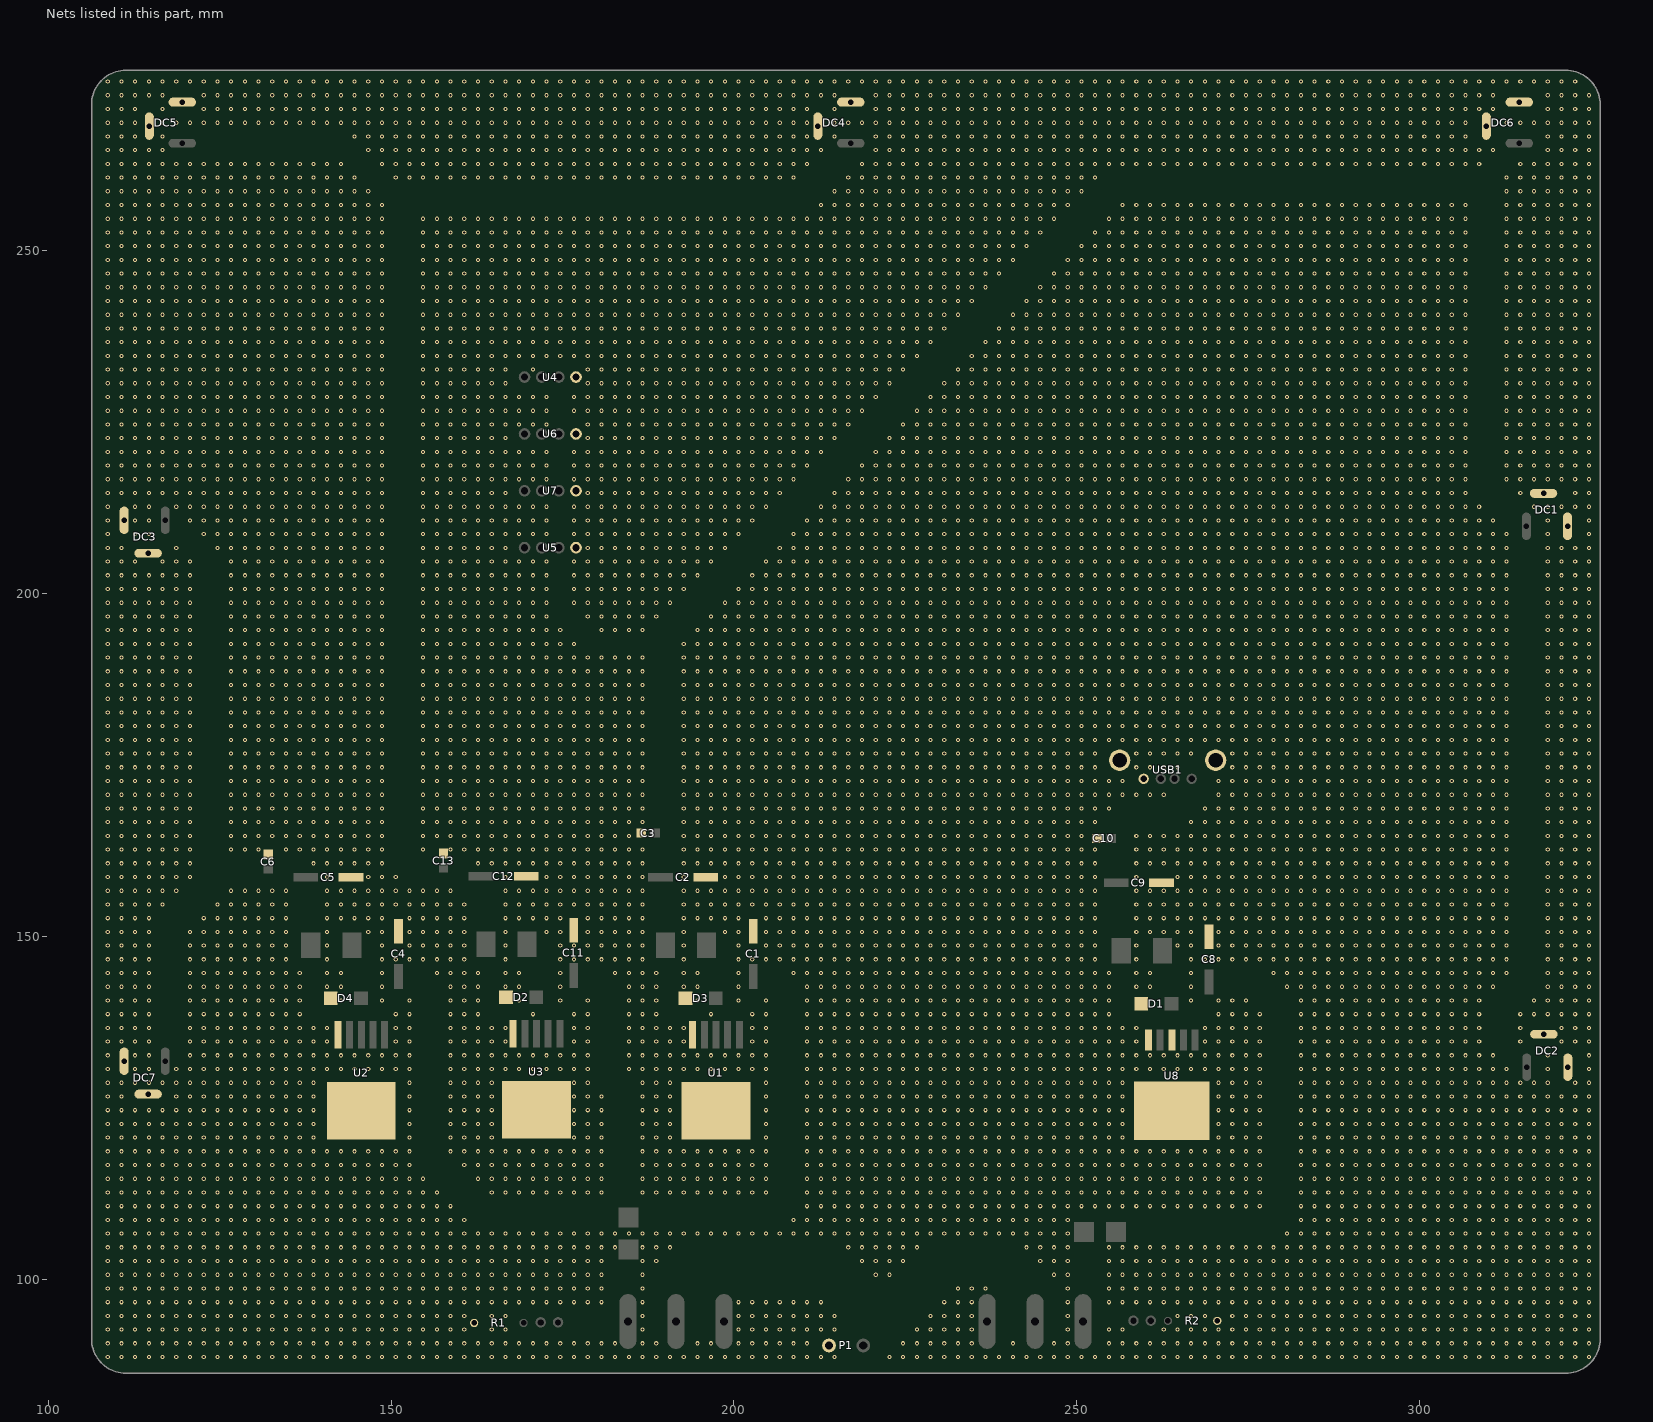
[diagram p0: the nets of this part, all layers, seen from the top]
# Altium PCB MISC49942.pcbdoc (part 4 of 4)
Units mm, origin at the board's own origin, x right, y up, seen from the top; angles counter-clockwise.
Board outline 220 x 190 mm, 2 copper layers (Top Layer, Bottom Layer), stack 1.58 mm thick; 45 components, 14 nets, 127 pads, 8689 vias.

## Via types
v1: diameter 0.61, hole 0.305, Top Layer to Bottom Layer, 8689 vias

## Nets (pads, with @x,y where several pads share a name; then routed paths per layer and width w, separated by ;. In a path a pad name is that pad's centre, name@x,y a point inside that pad or via, vN(x,y) a via of type N, cw(c..) or ccw(c..) an arc to the next point about the centre after c; other vN are vias at no path point) (continued)
GND: (continued)
  other v1: 204.684,220.669 206.684,220.669 208.684,220.669 210.684,220.669 212.684,220.669 220.684,220.669 222.684,220.669 224.684,220.669 226.684,220.669 228.684,220.669 230.684,220.669 232.684,220.669 234.684,220.669 236.684,220.669 238.684,220.669 240.684,220.669 242.684,220.669 244.684,220.669 246.684,220.669 248.684,220.669 250.684,220.669 252.684,220.669 254.684,220.669 256.684,220.669 258.684,220.669 260.684,220.669 262.684,220.669 264.684,220.669 266.684,220.669 268.684,220.669 270.684,220.669 272.684,220.669 274.684,220.669 276.684,220.669 278.684,220.669 280.684,220.669 282.684,220.669 284.684,220.669 286.684,220.669 288.684,220.669 290.684,220.669 292.684,220.669 294.684,220.669 296.684,220.669 298.684,220.669 300.684,220.669 302.684,220.669 304.684,220.669 306.684,220.669 312.684,220.669 314.684,220.669 316.684,220.669 318.684,220.669 320.684,220.669 322.684,220.669 324.684,220.669 108.684,222.669 110.684,222.669 112.684,222.669 114.684,222.669 116.684,222.669 118.684,222.669 120.684,222.669 122.684,222.669 124.684,222.669 126.684,222.669 128.684,222.669 130.684,222.669 132.684,222.669 134.684,222.669 136.684,222.669 138.684,222.669 140.684,222.669 142.684,222.669 144.684,222.669 146.684,222.669 148.684,222.669 154.684,222.669 156.684,222.669 158.684,222.669 160.684,222.669 162.684,222.669 164.684,222.669 166.684,222.669 178.684,222.669 180.684,222.669 182.684,222.669 184.684,222.669 186.684,222.669 188.684,222.669 190.684,222.669 192.684,222.669 194.684,222.669 196.684,222.669 198.684,222.669 200.684,222.669 202.684,222.669 204.684,222.669 206.684,222.669 208.684,222.669 210.684,222.669 212.684,222.669 214.684,222.669 222.684,222.669 224.684,222.669 226.684,222.669 228.684,222.669 230.684,222.669 232.684,222.669 234.684,222.669 236.684,222.669 238.684,222.669 240.684,222.669 242.684,222.669 244.684,222.669 246.684,222.669 248.684,222.669 250.684,222.669 252.684,222.669 254.684,222.669 256.684,222.669 258.684,222.669 260.684,222.669 262.684,222.669 264.684,222.669 266.684,222.669 268.684,222.669 270.684,222.669 272.684,222.669 274.684,222.669 276.684,222.669 278.684,222.669 280.684,222.669 282.684,222.669 284.684,222.669 286.684,222.669 288.684,222.669 290.684,222.669 292.684,222.669 294.684,222.669 296.684,222.669 298.684,222.669 300.684,222.669 302.684,222.669 304.684,222.669 306.684,222.669 312.684,222.669 314.684,222.669 316.684,222.669 318.684,222.669 320.684,222.669 322.684,222.669 324.684,222.669 108.684,224.669 110.684,224.669 112.684,224.669 114.684,224.669 116.684,224.669 118.684,224.669 120.684,224.669 122.684,224.669 124.684,224.669 126.684,224.669 128.684,224.669 130.684,224.669 132.684,224.669 134.684,224.669 136.684,224.669 138.684,224.669 140.684,224.669 142.684,224.669 144.684,224.669 146.684,224.669 148.684,224.669 154.684,224.669 156.684,224.669 158.684,224.669 160.684,224.669 162.684,224.669 164.684,224.669 166.684,224.669 168.684,224.669 170.684,224.669 172.684,224.669 178.684,224.669 180.684,224.669 182.684,224.669 184.684,224.669 186.684,224.669 188.684,224.669 190.684,224.669 192.684,224.669 194.684,224.669 196.684,224.669 198.684,224.669 200.684,224.669 202.684,224.669 204.684,224.669 206.684,224.669 208.684,224.669 210.684,224.669 212.684,224.669 214.684,224.669 216.684,224.669 224.684,224.669 226.684,224.669 228.684,224.669 230.684,224.669 232.684,224.669 234.684,224.669 236.684,224.669 238.684,224.669 240.684,224.669 242.684,224.669 244.684,224.669 246.684,224.669 248.684,224.669 250.684,224.669 252.684,224.669 254.684,224.669 256.684,224.669 258.684,224.669 260.684,224.669 262.684,224.669 264.684,224.669 266.684,224.669 268.684,224.669 270.684,224.669 272.684,224.669 274.684,224.669 276.684,224.669 278.684,224.669 280.684,224.669 282.684,224.669 284.684,224.669 286.684,224.669 288.684,224.669 290.684,224.669 292.684,224.669 294.684,224.669 296.684,224.669 298.684,224.669 300.684,224.669 302.684,224.669 304.684,224.669 306.684,224.669 312.684,224.669 314.684,224.669 316.684,224.669 318.684,224.669 320.684,224.669 322.684,224.669 324.684,224.669 108.684,226.669 110.684,226.669 112.684,226.669 114.684,226.669 116.684,226.669 118.684,226.669 120.684,226.669 122.684,226.669 124.684,226.669 126.684,226.669 128.684,226.669 130.684,226.669 132.684,226.669 134.684,226.669 136.684,226.669 138.684,226.669 140.684,226.669 142.684,226.669 144.684,226.669 146.684,226.669 148.684,226.669 154.684,226.669 156.684,226.669 158.684,226.669 160.684,226.669 162.684,226.669 164.684,226.669 166.684,226.669 168.684,226.669 170.684,226.669 172.684,226.669 176.684,226.669 178.684,226.669 180.684,226.669 182.684,226.669 184.684,226.669 186.684,226.669 188.684,226.669 190.684,226.669 192.684,226.669 194.684,226.669 196.684,226.669 198.684,226.669 200.684,226.669 202.684,226.669 204.684,226.669 206.684,226.669 208.684,226.669 210.684,226.669 212.684,226.669 214.684,226.669 216.684,226.669 218.684,226.669 226.684,226.669 228.684,226.669 230.684,226.669 232.684,226.669 234.684,226.669 236.684,226.669 238.684,226.669 240.684,226.669 242.684,226.669 244.684,226.669 246.684,226.669 248.684,226.669 250.684,226.669 252.684,226.669 254.684,226.669 256.684,226.669 258.684,226.669 260.684,226.669 262.684,226.669 264.684,226.669 266.684,226.669 268.684,226.669 270.684,226.669 272.684,226.669 274.684,226.669 276.684,226.669 278.684,226.669 280.684,226.669 282.684,226.669 284.684,226.669 286.684,226.669 288.684,226.669 290.684,226.669 292.684,226.669 294.684,226.669 296.684,226.669 298.684,226.669 300.684,226.669 302.684,226.669 304.684,226.669 306.684,226.669 312.684,226.669 314.684,226.669 316.684,226.669 318.684,226.669 320.684,226.669 322.684,226.669 324.684,226.669 108.684,228.669 110.684,228.669 112.684,228.669 114.684,228.669 116.684,228.669 118.684,228.669 120.684,228.669 122.684,228.669 124.684,228.669 126.684,228.669 128.684,228.669 130.684,228.669 132.684,228.669 134.684,228.669 136.684,228.669 138.684,228.669 140.684,228.669 142.684,228.669 144.684,228.669 146.684,228.669 148.684,228.669 154.684,228.669 156.684,228.669 158.684,228.669 160.684,228.669 162.684,228.669 164.684,228.669 166.684,228.669 168.684,228.669 170.684,228.669 172.684,228.669 176.684,228.669 178.684,228.669 180.684,228.669 182.684,228.669 184.684,228.669 186.684,228.669 188.684,228.669 190.684,228.669 192.684,228.669 194.684,228.669 196.684,228.669 198.684,228.669 200.684,228.669 202.684,228.669 204.684,228.669 206.684,228.669 208.684,228.669 210.684,228.669 212.684,228.669 214.684,228.669 216.684,228.669 218.684,228.669 220.684,228.669 228.684,228.669 230.684,228.669 232.684,228.669 234.684,228.669 236.684,228.669 238.684,228.669 240.684,228.669 242.684,228.669 244.684,228.669 246.684,228.669 248.684,228.669 250.684,228.669 252.684,228.669 254.684,228.669 256.684,228.669 258.684,228.669 260.684,228.669 262.684,228.669 264.684,228.669 266.684,228.669 268.684,228.669 270.684,228.669 272.684,228.669 274.684,228.669 276.684,228.669 278.684,228.669 280.684,228.669 282.684,228.669 284.684,228.669 286.684,228.669 288.684,228.669 290.684,228.669 292.684,228.669 294.684,228.669 296.684,228.669 298.684,228.669 300.684,228.669 302.684,228.669 304.684,228.669 306.684,228.669 312.684,228.669 314.684,228.669 316.684,228.669 318.684,228.669 320.684,228.669 322.684,228.669 324.684,228.669 108.684,230.669 110.684,230.669 112.684,230.669 114.684,230.669 116.684,230.669 118.684,230.669 120.684,230.669 122.684,230.669 124.684,230.669 126.684,230.669 128.684,230.669 130.684,230.669 132.684,230.669 134.684,230.669 136.684,230.669 138.684,230.669 140.684,230.669 142.684,230.669 144.684,230.669 146.684,230.669 148.684,230.669 154.684,230.669 156.684,230.669 158.684,230.669 160.684,230.669 162.684,230.669 164.684,230.669 166.684,230.669 178.684,230.669 180.684,230.669 182.684,230.669 184.684,230.669 186.684,230.669 188.684,230.669 190.684,230.669 192.684,230.669 194.684,230.669 196.684,230.669 198.684,230.669 200.684,230.669 202.684,230.669 204.684,230.669 206.684,230.669 208.684,230.669 210.684,230.669 212.684,230.669 214.684,230.669 216.684,230.669 218.684,230.669 220.684,230.669 222.684,230.669 230.684,230.669 232.684,230.669 234.684,230.669 236.684,230.669 238.684,230.669 240.684,230.669 242.684,230.669 244.684,230.669 246.684,230.669 248.684,230.669 250.684,230.669 252.684,230.669 254.684,230.669 256.684,230.669 258.684,230.669 260.684,230.669 262.684,230.669 264.684,230.669 266.684,230.669 268.684,230.669 270.684,230.669 272.684,230.669 274.684,230.669 276.684,230.669 278.684,230.669 280.684,230.669 282.684,230.669 284.684,230.669 286.684,230.669 288.684,230.669 290.684,230.669 292.684,230.669 294.684,230.669 296.684,230.669 298.684,230.669 300.684,230.669 302.684,230.669 304.684,230.669 306.684,230.669 312.684,230.669 314.684,230.669 316.684,230.669 318.684,230.669 320.684,230.669 322.684,230.669 324.684,230.669 108.684,232.669 110.684,232.669 112.684,232.669 114.684,232.669 116.684,232.669 118.684,232.669 120.684,232.669 122.684,232.669 124.684,232.669 126.684,232.669 128.684,232.669 130.684,232.669 132.684,232.669 134.684,232.669 136.684,232.669 138.684,232.669 140.684,232.669 142.684,232.669 144.684,232.669 146.684,232.669 148.684,232.669 154.684,232.669 156.684,232.669 158.684,232.669 160.684,232.669 162.684,232.669 164.684,232.669 166.684,232.669 170.684,232.669 178.684,232.669 180.684,232.669 182.684,232.669 184.684,232.669 186.684,232.669 188.684,232.669 190.684,232.669 192.684,232.669 194.684,232.669 196.684,232.669 198.684,232.669 200.684,232.669 202.684,232.669 204.684,232.669 206.684,232.669 208.684,232.669 210.684,232.669 212.684,232.669 214.684,232.669 216.684,232.669 218.684,232.669 220.684,232.669 222.684,232.669 224.684,232.669 232.684,232.669 234.684,232.669 236.684,232.669 238.684,232.669 240.684,232.669 242.684,232.669 244.684,232.669 246.684,232.669 248.684,232.669 250.684,232.669 252.684,232.669 254.684,232.669 256.684,232.669 258.684,232.669 260.684,232.669 262.684,232.669 264.684,232.669 266.684,232.669 268.684,232.669 270.684,232.669 272.684,232.669 274.684,232.669 276.684,232.669 278.684,232.669 280.684,232.669 282.684,232.669 284.684,232.669 286.684,232.669 288.684,232.669 290.684,232.669 292.684,232.669 294.684,232.669 296.684,232.669 298.684,232.669 300.684,232.669 302.684,232.669 304.684,232.669 306.684,232.669 312.684,232.669 314.684,232.669 316.684,232.669 318.684,232.669 320.684,232.669 322.684,232.669 324.684,232.669 108.684,234.669 110.684,234.669 112.684,234.669 114.684,234.669 116.684,234.669 118.684,234.669 120.684,234.669 122.684,234.669 124.684,234.669 126.684,234.669 128.684,234.669 130.684,234.669 132.684,234.669 134.684,234.669 136.684,234.669 138.684,234.669 140.684,234.669 142.684,234.669 144.684,234.669 146.684,234.669 148.684,234.669 154.684,234.669 156.684,234.669 158.684,234.669 160.684,234.669 162.684,234.669 164.684,234.669 166.684,234.669 168.684,234.669 170.684,234.669 172.684,234.669 174.684,234.669 176.684,234.669 178.684,234.669 180.684,234.669 182.684,234.669 184.684,234.669 186.684,234.669 188.684,234.669 190.684,234.669 192.684,234.669 194.684,234.669 196.684,234.669 198.684,234.669 200.684,234.669 202.684,234.669 204.684,234.669 206.684,234.669 208.684,234.669 210.684,234.669 212.684,234.669 214.684,234.669 216.684,234.669 218.684,234.669 220.684,234.669 222.684,234.669 224.684,234.669 226.684,234.669 234.684,234.669 236.684,234.669 238.684,234.669 240.684,234.669 242.684,234.669 244.684,234.669 246.684,234.669 248.684,234.669 250.684,234.669 252.684,234.669 254.684,234.669 256.684,234.669 258.684,234.669 260.684,234.669 262.684,234.669 264.684,234.669 266.684,234.669 268.684,234.669 270.684,234.669 272.684,234.669 274.684,234.669 276.684,234.669 278.684,234.669 280.684,234.669 282.684,234.669 284.684,234.669 286.684,234.669 288.684,234.669 290.684,234.669 292.684,234.669 294.684,234.669 296.684,234.669 298.684,234.669 300.684,234.669 302.684,234.669 304.684,234.669 306.684,234.669 312.684,234.669 314.684,234.669 316.684,234.669 318.684,234.669 320.684,234.669 322.684,234.669 324.684,234.669 108.684,236.669 110.684,236.669 112.684,236.669 114.684,236.669 116.684,236.669 118.684,236.669 120.684,236.669 122.684,236.669 124.684,236.669 126.684,236.669 128.684,236.669 130.684,236.669 132.684,236.669 134.684,236.669 136.684,236.669 138.684,236.669 140.684,236.669 142.684,236.669 144.684,236.669 146.684,236.669 148.684,236.669 154.684,236.669 156.684,236.669 158.684,236.669 160.684,236.669 162.684,236.669 164.684,236.669 166.684,236.669 168.684,236.669 170.684,236.669 172.684,236.669 174.684,236.669 176.684,236.669 178.684,236.669 180.684,236.669 182.684,236.669 184.684,236.669 186.684,236.669 188.684,236.669 190.684,236.669 192.684,236.669 194.684,236.669 196.684,236.669 198.684,236.669 200.684,236.669 202.684,236.669 204.684,236.669 206.684,236.669 208.684,236.669 210.684,236.669 212.684,236.669 214.684,236.669 216.684,236.669 218.684,236.669 220.684,236.669 222.684,236.669 224.684,236.669 226.684,236.669 228.684,236.669 236.684,236.669 238.684,236.669 240.684,236.669 242.684,236.669 244.684,236.669 246.684,236.669 248.684,236.669 250.684,236.669 252.684,236.669 254.684,236.669 256.684,236.669 258.684,236.669 260.684,236.669 262.684,236.669 264.684,236.669 266.684,236.669 268.684,236.669 270.684,236.669 272.684,236.669 274.684,236.669 276.684,236.669 278.684,236.669 280.684,236.669 282.684,236.669 284.684,236.669 286.684,236.669 288.684,236.669 290.684,236.669 292.684,236.669 294.684,236.669 296.684,236.669 298.684,236.669 300.684,236.669 302.684,236.669 304.684,236.669 306.684,236.669 312.684,236.669 314.684,236.669 316.684,236.669 318.684,236.669 320.684,236.669 322.684,236.669 324.684,236.669 108.684,238.669 110.684,238.669 112.684,238.669 114.684,238.669 116.684,238.669 118.684,238.669 120.684,238.669 122.684,238.669 124.684,238.669 126.684,238.669 128.684,238.669 130.684,238.669 132.684,238.669 134.684,238.669 136.684,238.669 138.684,238.669 140.684,238.669 142.684,238.669 144.684,238.669 146.684,238.669 148.684,238.669 154.684,238.669 156.684,238.669 158.684,238.669 160.684,238.669 162.684,238.669 164.684,238.669 166.684,238.669 168.684,238.669 170.684,238.669 172.684,238.669 174.684,238.669 176.684,238.669 178.684,238.669 180.684,238.669 182.684,238.669 184.684,238.669 186.684,238.669 188.684,238.669 190.684,238.669 192.684,238.669 194.684,238.669 196.684,238.669 198.684,238.669 200.684,238.669 202.684,238.669 204.684,238.669 206.684,238.669 208.684,238.669 210.684,238.669 212.684,238.669 214.684,238.669 216.684,238.669 218.684,238.669 220.684,238.669 222.684,238.669 224.684,238.669 226.684,238.669 228.684,238.669 230.684,238.669 238.684,238.669 240.684,238.669 242.684,238.669 244.684,238.669 246.684,238.669 248.684,238.669 250.684,238.669 252.684,238.669 254.684,238.669 256.684,238.669 258.684,238.669 260.684,238.669 262.684,238.669 264.684,238.669 266.684,238.669 268.684,238.669 270.684,238.669 272.684,238.669 274.684,238.669 276.684,238.669 278.684,238.669 280.684,238.669 282.684,238.669 284.684,238.669 286.684,238.669 288.684,238.669 290.684,238.669 292.684,238.669 294.684,238.669 296.684,238.669 298.684,238.669 300.684,238.669 302.684,238.669 304.684,238.669 306.684,238.669 312.684,238.669 314.684,238.669 316.684,238.669 318.684,238.669 320.684,238.669 322.684,238.669 324.684,238.669 108.684,240.669 110.684,240.669 112.684,240.669 114.684,240.669 116.684,240.669 118.684,240.669 120.684,240.669 122.684,240.669 124.684,240.669 126.684,240.669 128.684,240.669 130.684,240.669 132.684,240.669 134.684,240.669 136.684,240.669 138.684,240.669 140.684,240.669 142.684,240.669 144.684,240.669 146.684,240.669 148.684,240.669 154.684,240.669 156.684,240.669 158.684,240.669 160.684,240.669 162.684,240.669 164.684,240.669 166.684,240.669 168.684,240.669 170.684,240.669 172.684,240.669 174.684,240.669 176.684,240.669 178.684,240.669 180.684,240.669 182.684,240.669 184.684,240.669 186.684,240.669 188.684,240.669 190.684,240.669 192.684,240.669 194.684,240.669 196.684,240.669 198.684,240.669 200.684,240.669 202.684,240.669 204.684,240.669 206.684,240.669 208.684,240.669 210.684,240.669 212.684,240.669 214.684,240.669 216.684,240.669 218.684,240.669 220.684,240.669 222.684,240.669 224.684,240.669 226.684,240.669 228.684,240.669 230.684,240.669 232.684,240.669 240.684,240.669 242.684,240.669 244.684,240.669 246.684,240.669 248.684,240.669 250.684,240.669 252.684,240.669 254.684,240.669 256.684,240.669 258.684,240.669 260.684,240.669 262.684,240.669 264.684,240.669 266.684,240.669 268.684,240.669 270.684,240.669 272.684,240.669 274.684,240.669 276.684,240.669 278.684,240.669 280.684,240.669 282.684,240.669 284.684,240.669 286.684,240.669 288.684,240.669 290.684,240.669 292.684,240.669 294.684,240.669 296.684,240.669 298.684,240.669 300.684,240.669 302.684,240.669 304.684,240.669 306.684,240.669 312.684,240.669 314.684,240.669 316.684,240.669 318.684,240.669 320.684,240.669 322.684,240.669 324.684,240.669 108.684,242.669 110.684,242.669 112.684,242.669 114.684,242.669 116.684,242.669 118.684,242.669 120.684,242.669 122.684,242.669 124.684,242.669 126.684,242.669 128.684,242.669 130.684,242.669 132.684,242.669 134.684,242.669 136.684,242.669 138.684,242.669 140.684,242.669 142.684,242.669 144.684,242.669 146.684,242.669 148.684,242.669 154.684,242.669 156.684,242.669 158.684,242.669 160.684,242.669 162.684,242.669 164.684,242.669 166.684,242.669 168.684,242.669 170.684,242.669 172.684,242.669 174.684,242.669 176.684,242.669 178.684,242.669 180.684,242.669 182.684,242.669 184.684,242.669 186.684,242.669 188.684,242.669 190.684,242.669 192.684,242.669 194.684,242.669 196.684,242.669 198.684,242.669 200.684,242.669 202.684,242.669 204.684,242.669 206.684,242.669 208.684,242.669 210.684,242.669 212.684,242.669 214.684,242.669 216.684,242.669 218.684,242.669 220.684,242.669 222.684,242.669 224.684,242.669 226.684,242.669 228.684,242.669 230.684,242.669 232.684,242.669 234.684,242.669 242.684,242.669 244.684,242.669 246.684,242.669 248.684,242.669 250.684,242.669 252.684,242.669 254.684,242.669 256.684,242.669 258.684,242.669 260.684,242.669 262.684,242.669 264.684,242.669 266.684,242.669 268.684,242.669 270.684,242.669 272.684,242.669 274.684,242.669 276.684,242.669 278.684,242.669 280.684,242.669 282.684,242.669 284.684,242.669 286.684,242.669 288.684,242.669 290.684,242.669 292.684,242.669 294.684,242.669 296.684,242.669 298.684,242.669 300.684,242.669 302.684,242.669 304.684,242.669 306.684,242.669 312.684,242.669 314.684,242.669 316.684,242.669 318.684,242.669 320.684,242.669 322.684,242.669 324.684,242.669 108.684,244.669 110.684,244.669 112.684,244.669 114.684,244.669 116.684,244.669 118.684,244.669 120.684,244.669 122.684,244.669 124.684,244.669 126.684,244.669 128.684,244.669 130.684,244.669 132.684,244.669 134.684,244.669 136.684,244.669 138.684,244.669 140.684,244.669 142.684,244.669 144.684,244.669 146.684,244.669 148.684,244.669 154.684,244.669 156.684,244.669 158.684,244.669 160.684,244.669 162.684,244.669 164.684,244.669 166.684,244.669 168.684,244.669 170.684,244.669 172.684,244.669 174.684,244.669 176.684,244.669 178.684,244.669 180.684,244.669 182.684,244.669 184.684,244.669 186.684,244.669 188.684,244.669 190.684,244.669 192.684,244.669 194.684,244.669 196.684,244.669 198.684,244.669 200.684,244.669 202.684,244.669 204.684,244.669 206.684,244.669 208.684,244.669 210.684,244.669 212.684,244.669 214.684,244.669 216.684,244.669 218.684,244.669 220.684,244.669 222.684,244.669 224.684,244.669 226.684,244.669 228.684,244.669 230.684,244.669 232.684,244.669 234.684,244.669 236.684,244.669 244.684,244.669 246.684,244.669 248.684,244.669 250.684,244.669 252.684,244.669 254.684,244.669 256.684,244.669 258.684,244.669 260.684,244.669 262.684,244.669 264.684,244.669 266.684,244.669 268.684,244.669 270.684,244.669 272.684,244.669 274.684,244.669 276.684,244.669 278.684,244.669 280.684,244.669 282.684,244.669 284.684,244.669 286.684,244.669 288.684,244.669 290.684,244.669 292.684,244.669 294.684,244.669 296.684,244.669 298.684,244.669 300.684,244.669 302.684,244.669 304.684,244.669 306.684,244.669 312.684,244.669 314.684,244.669 316.684,244.669 318.684,244.669 320.684,244.669 322.684,244.669 324.684,244.669 108.684,246.669 110.684,246.669 112.684,246.669 114.684,246.669 116.684,246.669 118.684,246.669 120.684,246.669 122.684,246.669 124.684,246.669 126.684,246.669 128.684,246.669 130.684,246.669 132.684,246.669 134.684,246.669 136.684,246.669 138.684,246.669 140.684,246.669 142.684,246.669 144.684,246.669 146.684,246.669 148.684,246.669 154.684,246.669 156.684,246.669 158.684,246.669 160.684,246.669 162.684,246.669 164.684,246.669 166.684,246.669 168.684,246.669 170.684,246.669 172.684,246.669 174.684,246.669 176.684,246.669 178.684,246.669 180.684,246.669 182.684,246.669 184.684,246.669 186.684,246.669 188.684,246.669 190.684,246.669 192.684,246.669 194.684,246.669 196.684,246.669 198.684,246.669 200.684,246.669 202.684,246.669 204.684,246.669 206.684,246.669 208.684,246.669 210.684,246.669 212.684,246.669 214.684,246.669 216.684,246.669 218.684,246.669 220.684,246.669 222.684,246.669 224.684,246.669 226.684,246.669 228.684,246.669 230.684,246.669 232.684,246.669 234.684,246.669 236.684,246.669 238.684,246.669 246.684,246.669 248.684,246.669 250.684,246.669 252.684,246.669 254.684,246.669 256.684,246.669 258.684,246.669 260.684,246.669 262.684,246.669 264.684,246.669 266.684,246.669 268.684,246.669 270.684,246.669 272.684,246.669 274.684,246.669 276.684,246.669 278.684,246.669 280.684,246.669 282.684,246.669 284.684,246.669 286.684,246.669 288.684,246.669 290.684,246.669 292.684,246.669 294.684,246.669 296.684,246.669 298.684,246.669 300.684,246.669 302.684,246.669 304.684,246.669 306.684,246.669 312.684,246.669 314.684,246.669 316.684,246.669 318.684,246.669 320.684,246.669 322.684,246.669 324.684,246.669 108.684,248.669 110.684,248.669 112.684,248.669 114.684,248.669 116.684,248.669 118.684,248.669 120.684,248.669 122.684,248.669 124.684,248.669 126.684,248.669 128.684,248.669 130.684,248.669 132.684,248.669 134.684,248.669 136.684,248.669 138.684,248.669 140.684,248.669 142.684,248.669 144.684,248.669 146.684,248.669 148.684,248.669 154.684,248.669 156.684,248.669 158.684,248.669 160.684,248.669 162.684,248.669 164.684,248.669 166.684,248.669 168.684,248.669 170.684,248.669 172.684,248.669 174.684,248.669 176.684,248.669 178.684,248.669 180.684,248.669 182.684,248.669 184.684,248.669 186.684,248.669 188.684,248.669 190.684,248.669 192.684,248.669 194.684,248.669 196.684,248.669 198.684,248.669 200.684,248.669 202.684,248.669 204.684,248.669 206.684,248.669 208.684,248.669 210.684,248.669 212.684,248.669 214.684,248.669 216.684,248.669 218.684,248.669 220.684,248.669 222.684,248.669 224.684,248.669 226.684,248.669 228.684,248.669 230.684,248.669 232.684,248.669 234.684,248.669 236.684,248.669 238.684,248.669 240.684,248.669 248.684,248.669 250.684,248.669 252.684,248.669 254.684,248.669 256.684,248.669 258.684,248.669 260.684,248.669 262.684,248.669 264.684,248.669 266.684,248.669 268.684,248.669 270.684,248.669 272.684,248.669 274.684,248.669 276.684,248.669 278.684,248.669 280.684,248.669 282.684,248.669 284.684,248.669 286.684,248.669 288.684,248.669 290.684,248.669 292.684,248.669 294.684,248.669 296.684,248.669 298.684,248.669 300.684,248.669 302.684,248.669 304.684,248.669 306.684,248.669 312.684,248.669 314.684,248.669 316.684,248.669 318.684,248.669 320.684,248.669 322.684,248.669 324.684,248.669 108.684,250.669 110.684,250.669 112.684,250.669 114.684,250.669 116.684,250.669 118.684,250.669 120.684,250.669 122.684,250.669 124.684,250.669 126.684,250.669 128.684,250.669 130.684,250.669 132.684,250.669 134.684,250.669 136.684,250.669 138.684,250.669 140.684,250.669 142.684,250.669 144.684,250.669 146.684,250.669 148.684,250.669 154.684,250.669 156.684,250.669 158.684,250.669 160.684,250.669 162.684,250.669 164.684,250.669 166.684,250.669 168.684,250.669 170.684,250.669 172.684,250.669 174.684,250.669 176.684,250.669 178.684,250.669 180.684,250.669 182.684,250.669 184.684,250.669 186.684,250.669 188.684,250.669 190.684,250.669 192.684,250.669 194.684,250.669 196.684,250.669 198.684,250.669 200.684,250.669 202.684,250.669 204.684,250.669 206.684,250.669 208.684,250.669 210.684,250.669 212.684,250.669 214.684,250.669 216.684,250.669 218.684,250.669 220.684,250.669 222.684,250.669 224.684,250.669 226.684,250.669 228.684,250.669 230.684,250.669 232.684,250.669 234.684,250.669 236.684,250.669 238.684,250.669 240.684,250.669 242.684,250.669 250.684,250.669 252.684,250.669 254.684,250.669 256.684,250.669 258.684,250.669 260.684,250.669 262.684,250.669 264.684,250.669 266.684,250.669 268.684,250.669 270.684,250.669 272.684,250.669 274.684,250.669 276.684,250.669 278.684,250.669 280.684,250.669 282.684,250.669 284.684,250.669 286.684,250.669 288.684,250.669 290.684,250.669 292.684,250.669 294.684,250.669 296.684,250.669 298.684,250.669 300.684,250.669 302.684,250.669 304.684,250.669 306.684,250.669 312.684,250.669 314.684,250.669 316.684,250.669 318.684,250.669 320.684,250.669 322.684,250.669 324.684,250.669 108.684,252.669 110.684,252.669 112.684,252.669 114.684,252.669 116.684,252.669 118.684,252.669 120.684,252.669 122.684,252.669 124.684,252.669 126.684,252.669 128.684,252.669 130.684,252.669 132.684,252.669 134.684,252.669 136.684,252.669 138.684,252.669 140.684,252.669 142.684,252.669 144.684,252.669 146.684,252.669 148.684,252.669 154.684,252.669 156.684,252.669 158.684,252.669 160.684,252.669 162.684,252.669 164.684,252.669 166.684,252.669 168.684,252.669 170.684,252.669 172.684,252.669 174.684,252.669 176.684,252.669 178.684,252.669 180.684,252.669 182.684,252.669 184.684,252.669 186.684,252.669 188.684,252.669 190.684,252.669 192.684,252.669 194.684,252.669 196.684,252.669 198.684,252.669 200.684,252.669 202.684,252.669 204.684,252.669 206.684,252.669 208.684,252.669 210.684,252.669 212.684,252.669 214.684,252.669 216.684,252.669 218.684,252.669 220.684,252.669 222.684,252.669 224.684,252.669 226.684,252.669 228.684,252.669 230.684,252.669 232.684,252.669 234.684,252.669 236.684,252.669 238.684,252.669 240.684,252.669 242.684,252.669 244.684,252.669 252.684,252.669 254.684,252.669 256.684,252.669 258.684,252.669 260.684,252.669 262.684,252.669 264.684,252.669 266.684,252.669 268.684,252.669 270.684,252.669 272.684,252.669 274.684,252.669 276.684,252.669 278.684,252.669 280.684,252.669 282.684,252.669 284.684,252.669 286.684,252.669 288.684,252.669 290.684,252.669 292.684,252.669 294.684,252.669 296.684,252.669 298.684,252.669 300.684,252.669 302.684,252.669 304.684,252.669 306.684,252.669 312.684,252.669 314.684,252.669 316.684,252.669 318.684,252.669 320.684,252.669 322.684,252.669 324.684,252.669 108.684,254.669 110.684,254.669 112.684,254.669 114.684,254.669 116.684,254.669 118.684,254.669 120.684,254.669 122.684,254.669 124.684,254.669 126.684,254.669 128.684,254.669 130.684,254.669 132.684,254.669 134.684,254.669 136.684,254.669 138.684,254.669 140.684,254.669 142.684,254.669 144.684,254.669 146.684,254.669 148.684,254.669 154.684,254.669 156.684,254.669 158.684,254.669 160.684,254.669 162.684,254.669 164.684,254.669 166.684,254.669 168.684,254.669 170.684,254.669 172.684,254.669 174.684,254.669 176.684,254.669 178.684,254.669 180.684,254.669 182.684,254.669 184.684,254.669 186.684,254.669 188.684,254.669 190.684,254.669 192.684,254.669 194.684,254.669 196.684,254.669 198.684,254.669 200.684,254.669 202.684,254.669 204.684,254.669 206.684,254.669 208.684,254.669 210.684,254.669 212.684,254.669 214.684,254.669 216.684,254.669 218.684,254.669 220.684,254.669 222.684,254.669 224.684,254.669 226.684,254.669 228.684,254.669 230.684,254.669 232.684,254.669 234.684,254.669 236.684,254.669 238.684,254.669 240.684,254.669 242.684,254.669 244.684,254.669 246.684,254.669 254.684,254.669 256.684,254.669 258.684,254.669 260.684,254.669 262.684,254.669 264.684,254.669 266.684,254.669 268.684,254.669 270.684,254.669 272.684,254.669 274.684,254.669 276.684,254.669 278.684,254.669 280.684,254.669 282.684,254.669 284.684,254.669 286.684,254.669 288.684,254.669 290.684,254.669 292.684,254.669 294.684,254.669 296.684,254.669 298.684,254.669 300.684,254.669 302.684,254.669 304.684,254.669 306.684,254.669 312.684,254.669 314.684,254.669 316.684,254.669 318.684,254.669 320.684,254.669 322.684,254.669 324.684,254.669 108.684,256.669 110.684,256.669 112.684,256.669 114.684,256.669 116.684,256.669 118.684,256.669 120.684,256.669 122.684,256.669 124.684,256.669 126.684,256.669 128.684,256.669 130.684,256.669 132.684,256.669 134.684,256.669 136.684,256.669 138.684,256.669 140.684,256.669 142.684,256.669 144.684,256.669 146.684,256.669 148.684,256.669 212.684,256.669 214.684,256.669 216.684,256.669 218.684,256.669 220.684,256.669 222.684,256.669 224.684,256.669 226.684,256.669 228.684,256.669 230.684,256.669 232.684,256.669 234.684,256.669 236.684,256.669 238.684,256.669 240.684,256.669 242.684,256.669 244.684,256.669 246.684,256.669 248.684,256.669 256.684,256.669 258.684,256.669 260.684,256.669 262.684,256.669 264.684,256.669 266.684,256.669 268.684,256.669 270.684,256.669 272.684,256.669 274.684,256.669 276.684,256.669 278.684,256.669 280.684,256.669 282.684,256.669 284.684,256.669 286.684,256.669 288.684,256.669 290.684,256.669 292.684,256.669 294.684,256.669 296.684,256.669 298.684,256.669 300.684,256.669 302.684,256.669 304.684,256.669 306.684,256.669 312.684,256.669 314.684,256.669 316.684,256.669 318.684,256.669 320.684,256.669 322.684,256.669 324.684,256.669 108.684,258.669 110.684,258.669 112.684,258.669 114.684,258.669 116.684,258.669 118.684,258.669 120.684,258.669 122.684,258.669 124.684,258.669 126.684,258.669 128.684,258.669 130.684,258.669 132.684,258.669 134.684,258.669 136.684,258.669 138.684,258.669 140.684,258.669 142.684,258.669 144.684,258.669 146.684,258.669 214.684,258.669 216.684,258.669 218.684,258.669 220.684,258.669 222.684,258.669 224.684,258.669 226.684,258.669 228.684,258.669 230.684,258.669 232.684,258.669 234.684,258.669 236.684,258.669 238.684,258.669 240.684,258.669 242.684,258.669 244.684,258.669 246.684,258.669 248.684,258.669 250.684,258.669 312.684,258.669 314.684,258.669 316.684,258.669 318.684,258.669 320.684,258.669 322.684,258.669 324.684,258.669 108.684,260.669 110.684,260.669 112.684,260.669 114.684,260.669 116.684,260.669 118.684,260.669 120.684,260.669 122.684,260.669 124.684,260.669 126.684,260.669 128.684,260.669 130.684,260.669 132.684,260.669 134.684,260.669 136.684,260.669 138.684,260.669 140.684,260.669 142.684,260.669 144.684,260.669 150.684,260.669 152.684,260.669 154.684,260.669 156.684,260.669 158.684,260.669 160.684,260.669 162.684,260.669 164.684,260.669 166.684,260.669 168.684,260.669 170.684,260.669 172.684,260.669 174.684,260.669 176.684,260.669 178.684,260.669 180.684,260.669 182.684,260.669 184.684,260.669 186.684,260.669 188.684,260.669 190.684,260.669 192.684,260.669 194.684,260.669 196.684,260.669 198.684,260.669 200.684,260.669 202.684,260.669 204.684,260.669 206.684,260.669 208.684,260.669 216.684,260.669 218.684,260.669 220.684,260.669 222.684,260.669 224.684,260.669 226.684,260.669 228.684,260.669 230.684,260.669 232.684,260.669 234.684,260.669 236.684,260.669 238.684,260.669 240.684,260.669 242.684,260.669 244.684,260.669 246.684,260.669 248.684,260.669 250.684,260.669 252.684,260.669 312.684,260.669 314.684,260.669 316.684,260.669 318.684,260.669 320.684,260.669 322.684,260.669 324.684,260.669 108.684,262.669 110.684,262.669 112.684,262.669 114.684,262.669 116.684,262.669 118.684,262.669 120.684,262.669 122.684,262.669 124.684,262.669 126.684,262.669 128.684,262.669 130.684,262.669 132.684,262.669 134.684,262.669 136.684,262.669 138.684,262.669 140.684,262.669 142.684,262.669 148.684,262.669 150.684,262.669 152.684,262.669 154.684,262.669 156.684,262.669 158.684,262.669 160.684,262.669 162.684,262.669 164.684,262.669 166.684,262.669 168.684,262.669 170.684,262.669 172.684,262.669 174.684,262.669 176.684,262.669 178.684,262.669 180.684,262.669 182.684,262.669 184.684,262.669 186.684,262.669 188.684,262.669 190.684,262.669 192.684,262.669 194.684,262.669 196.684,262.669 198.684,262.669 200.684,262.669 202.684,262.669 204.684,262.669 206.684,262.669 208.684,262.669 210.684,262.669 218.684,262.669 220.684,262.669 222.684,262.669 224.684,262.669 226.684,262.669 228.684,262.669 230.684,262.669 232.684,262.669 234.684,262.669 236.684,262.669 238.684,262.669 240.684,262.669 242.684,262.669 244.684,262.669 246.684,262.669 248.684,262.669 250.684,262.669 252.684,262.669 254.684,262.669 256.684,262.669 258.684,262.669 260.684,262.669 262.684,262.669 264.684,262.669 266.684,262.669 268.684,262.669 270.684,262.669 272.684,262.669 274.684,262.669 276.684,262.669 278.684,262.669 280.684,262.669 282.684,262.669 284.684,262.669 286.684,262.669 288.684,262.669 290.684,262.669 292.684,262.669 294.684,262.669 296.684,262.669 298.684,262.669 300.684,262.669 302.684,262.669 304.684,262.669 306.684,262.669 308.684,262.669 314.684,262.669 316.684,262.669 318.684,262.669 320.684,262.669 322.684,262.669 324.684,262.669 108.684,264.669 110.684,264.669 112.684,264.669 114.684,264.669 116.684,264.669 146.684,264.669 148.684,264.669 150.684,264.669 152.684,264.669 154.684,264.669 156.684,264.669 158.684,264.669 160.684,264.669 162.684,264.669 164.684,264.669 166.684,264.669 168.684,264.669 170.684,264.669 172.684,264.669 174.684,264.669 176.684,264.669 178.684,264.669 180.684,264.669 182.684,264.669 184.684,264.669 186.684,264.669 188.684,264.669 190.684,264.669 192.684,264.669 194.684,264.669 196.684,264.669 198.684,264.669 200.684,264.669 202.684,264.669 204.684,264.669 206.684,264.669 208.684,264.669 210.684,264.669 212.684,264.669 220.684,264.669 222.684,264.669 224.684,264.669 226.684,264.669 228.684,264.669 230.684,264.669 232.684,264.669 234.684,264.669 236.684,264.669 238.684,264.669 240.684,264.669 242.684,264.669 244.684,264.669 246.684,264.669 248.684,264.669 250.684,264.669 252.684,264.669 254.684,264.669 256.684,264.669 258.684,264.669 260.684,264.669 262.684,264.669 264.684,264.669 266.684,264.669 268.684,264.669 270.684,264.669 272.684,264.669 274.684,264.669 276.684,264.669 278.684,264.669 280.684,264.669 282.684,264.669 284.684,264.669 286.684,264.669 288.684,264.669 290.684,264.669 292.684,264.669 294.684,264.669 296.684,264.669 298.684,264.669 300.684,264.669 302.684,264.669 304.684,264.669 306.684,264.669 308.684,264.669 310.684,264.669 318.684,264.669 320.684,264.669 322.684,264.669 324.684,264.669 108.684,266.669 110.684,266.669 112.684,266.669 116.684,266.669 144.684,266.669 146.684,266.669 148.684,266.669 150.684,266.669 152.684,266.669 154.684,266.669 156.684,266.669 158.684,266.669 160.684,266.669 162.684,266.669 164.684,266.669 166.684,266.669 168.684,266.669 170.684,266.669 172.684,266.669 174.684,266.669 176.684,266.669 178.684,266.669 180.684,266.669 182.684,266.669 184.684,266.669 186.684,266.669 188.684,266.669 190.684,266.669 192.684,266.669 194.684,266.669 196.684,266.669 198.684,266.669 200.684,266.669 202.684,266.669 204.684,266.669 206.684,266.669 208.684,266.669 210.684,266.669 214.684,266.669 220.684,266.669 222.684,266.669 224.684,266.669 226.684,266.669 228.684,266.669 230.684,266.669 232.684,266.669 234.684,266.669 236.684,266.669 238.684,266.669 240.684,266.669 242.684,266.669 244.684,266.669 246.684,266.669 248.684,266.669 250.684,266.669 252.684,266.669 254.684,266.669 256.684,266.669 258.684,266.669 260.684,266.669 262.684,266.669 264.684,266.669 266.684,266.669 268.684,266.669 270.684,266.669 272.684,266.669 274.684,266.669 276.684,266.669 278.684,266.669 280.684,266.669 282.684,266.669 284.684,266.669 286.684,266.669 288.684,266.669 290.684,266.669 292.684,266.669 294.684,266.669 296.684,266.669 298.684,266.669 300.684,266.669 302.684,266.669 304.684,266.669 306.684,266.669 318.684,266.669 320.684,266.669 322.684,266.669 324.684,266.669 108.684,268.669 110.684,268.669 112.684,268.669 116.684,268.669 118.684,268.669 120.684,268.669 122.684,268.669 124.684,268.669 126.684,268.669 128.684,268.669 130.684,268.669 132.684,268.669 134.684,268.669 136.684,268.669 138.684,268.669 140.684,268.669 142.684,268.669 144.684,268.669 146.684,268.669 148.684,268.669 150.684,268.669 152.684,268.669 154.684,268.669 156.684,268.669 158.684,268.669 160.684,268.669 162.684,268.669 164.684,268.669 166.684,268.669 168.684,268.669 170.684,268.669 172.684,268.669 174.684,268.669 176.684,268.669 178.684,268.669 180.684,268.669 182.684,268.669 184.684,268.669 186.684,268.669 188.684,268.669 190.684,268.669 192.684,268.669 194.684,268.669 196.684,268.669 198.684,268.669 200.684,268.669 202.684,268.669 204.684,268.669 206.684,268.669 208.684,268.669 210.684,268.669 214.684,268.669 216.684,268.669 218.684,268.669 220.684,268.669 222.684,268.669 224.684,268.669 226.684,268.669 228.684,268.669 230.684,268.669 232.684,268.669 234.684,268.669 236.684,268.669 238.684,268.669 240.684,268.669 242.684,268.669 244.684,268.669 246.684,268.669 248.684,268.669 250.684,268.669 252.684,268.669 254.684,268.669 256.684,268.669 258.684,268.669 260.684,268.669 262.684,268.669 264.684,268.669 266.684,268.669 268.684,268.669 270.684,268.669 272.684,268.669 274.684,268.669 276.684,268.669 278.684,268.669 280.684,268.669 282.684,268.669 284.684,268.669 286.684,268.669 288.684,268.669 290.684,268.669 292.684,268.669 294.684,268.669 296.684,268.669 298.684,268.669 300.684,268.669 302.684,268.669 304.684,268.669 306.684,268.669 312.684,268.669 314.684,268.669 316.684,268.669 318.684,268.669 320.684,268.669 322.684,268.669 324.684,268.669 108.684,270.669 110.684,270.669 112.684,270.669 116.684,270.669 122.684,270.669 124.684,270.669 126.684,270.669 128.684,270.669 130.684,270.669 132.684,270.669 134.684,270.669 136.684,270.669 138.684,270.669 140.684,270.669 142.684,270.669 144.684,270.669 146.684,270.669 148.684,270.669 150.684,270.669 152.684,270.669 154.684,270.669 156.684,270.669 158.684,270.669 160.684,270.669 162.684,270.669 164.684,270.669 166.684,270.669 168.684,270.669 170.684,270.669 172.684,270.669 174.684,270.669 176.684,270.669 178.684,270.669 180.684,270.669 182.684,270.669 184.684,270.669 186.684,270.669 188.684,270.669 190.684,270.669 192.684,270.669 194.684,270.669 196.684,270.669 198.684,270.669 200.684,270.669 202.684,270.669 204.684,270.669 206.684,270.669 208.684,270.669 210.684,270.669 214.684,270.669 220.684,270.669 222.684,270.669 224.684,270.669 226.684,270.669 228.684,270.669 230.684,270.669 232.684,270.669 234.684,270.669 236.684,270.669 238.684,270.669 240.684,270.669 242.684,270.669 244.684,270.669 246.684,270.669 248.684,270.669 250.684,270.669 252.684,270.669 254.684,270.669 256.684,270.669 258.684,270.669 260.684,270.669 262.684,270.669 264.684,270.669 266.684,270.669 268.684,270.669 270.684,270.669 272.684,270.669 274.684,270.669 276.684,270.669 278.684,270.669 280.684,270.669 282.684,270.669 284.684,270.669 286.684,270.669 288.684,270.669 290.684,270.669 292.684,270.669 294.684,270.669 296.684,270.669 298.684,270.669 300.684,270.669 302.684,270.669 304.684,270.669 306.684,270.669 308.684,270.669 310.684,270.669 318.684,270.669 320.684,270.669 322.684,270.669 324.684,270.669 108.684,272.669 110.684,272.669 112.684,272.669 114.684,272.669 116.684,272.669 122.684,272.669 124.684,272.669 126.684,272.669 128.684,272.669 130.684,272.669 132.684,272.669 134.684,272.669 136.684,272.669 138.684,272.669 140.684,272.669 142.684,272.669 144.684,272.669 146.684,272.669 148.684,272.669 150.684,272.669 152.684,272.669 154.684,272.669 156.684,272.669 158.684,272.669 160.684,272.669 162.684,272.669 164.684,272.669 166.684,272.669 168.684,272.669 170.684,272.669 172.684,272.669 174.684,272.669 176.684,272.669 178.684,272.669 180.684,272.669 182.684,272.669 184.684,272.669 186.684,272.669 188.684,272.669 190.684,272.669 192.684,272.669 194.684,272.669 196.684,272.669 198.684,272.669 200.684,272.669 202.684,272.669 204.684,272.669 206.684,272.669 208.684,272.669 210.684,272.669 212.684,272.669 214.684,272.669 220.684,272.669 222.684,272.669 224.684,272.669 226.684,272.669 228.684,272.669 230.684,272.669 232.684,272.669 234.684,272.669 236.684,272.669 238.684,272.669 240.684,272.669 242.684,272.669 244.684,272.669 246.684,272.669 248.684,272.669 250.684,272.669 252.684,272.669 254.684,272.669 256.684,272.669 258.684,272.669 260.684,272.669 262.684,272.669 264.684,272.669 266.684,272.669 268.684,272.669 270.684,272.669 272.684,272.669 274.684,272.669 276.684,272.669 278.684,272.669 280.684,272.669 282.684,272.669 284.684,272.669 286.684,272.669 288.684,272.669 290.684,272.669 292.684,272.669 294.684,272.669 296.684,272.669 298.684,272.669 300.684,272.669 302.684,272.669 304.684,272.669 306.684,272.669 308.684,272.669 310.684,272.669 318.684,272.669 320.684,272.669 322.684,272.669 324.684,272.669 108.684,274.669 110.684,274.669 112.684,274.669 114.684,274.669 116.684,274.669 118.684,274.669 120.684,274.669 122.684,274.669 124.684,274.669 126.684,274.669 128.684,274.669 130.684,274.669 132.684,274.669 134.684,274.669 136.684,274.669 138.684,274.669 140.684,274.669 142.684,274.669 144.684,274.669 146.684,274.669 148.684,274.669 150.684,274.669 152.684,274.669 154.684,274.669 156.684,274.669 158.684,274.669 160.684,274.669 162.684,274.669 164.684,274.669 166.684,274.669 168.684,274.669 170.684,274.669 172.684,274.669 174.684,274.669 176.684,274.669 178.684,274.669 180.684,274.669 182.684,274.669 184.684,274.669 186.684,274.669 188.684,274.669 190.684,274.669 192.684,274.669 194.684,274.669 196.684,274.669 198.684,274.669 200.684,274.669 202.684,274.669 204.684,274.669 206.684,274.669 208.684,274.669 210.684,274.669 212.684,274.669 214.684,274.669 216.684,274.669 218.684,274.669 220.684,274.669 222.684,274.669 224.684,274.669 226.684,274.669 228.684,274.669 230.684,274.669 232.684,274.669 234.684,274.669 236.684,274.669 238.684,274.669 240.684,274.669 242.684,274.669 244.684,274.669 246.684,274.669 248.684,274.669 250.684,274.669 252.684,274.669 254.684,274.669 256.684,274.669 258.684,274.669 260.684,274.669 262.684,274.669 264.684,274.669 266.684,274.669 268.684,274.669 270.684,274.669 272.684,274.669 274.684,274.669 276.684,274.669 278.684,274.669 280.684,274.669 282.684,274.669 284.684,274.669 286.684,274.669 288.684,274.669 290.684,274.669 292.684,274.669 294.684,274.669 296.684,274.669 298.684,274.669 300.684,274.669 302.684,274.669 304.684,274.669 306.684,274.669 308.684,274.669 310.684,274.669 312.684,274.669 314.684,274.669 316.684,274.669 318.684,274.669 320.684,274.669 322.684,274.669
pads on no net: SW1.1 SW2.1 U1.3 U2.3 U3.3 U4.3 U4.4 U5.3 U5.4 U6.3 U6.4 U7.3 U7.4 USB1.2 USB1.3

## Polygon pours and split planes (outlines as drawn)
GND on Top Layer (solid, remove dead copper, pour order 0): 94.075,285.175 94.075,76.2 352.225,76.2 352.225,285.175
GND on Bottom Layer (solid, remove dead copper, pour order 2): 76.2,285.9 76.2,82.575 352.35,82.575 352.35,285.9

## Keep-outs
Top Layer:
  region: 163.692,145.677 170.181,145.677 170.181,151.989 163.692,151.989
  region: 138.142,145.527 144.631,145.527 144.631,151.839 138.142,151.839
  region: 189.867,145.527 196.356,145.527 196.356,151.839 189.867,151.839
  region: 256.34,144.748 262.83,144.748 262.83,151.06 256.34,151.06
Board Outline Layer:
  the board outline again, w0.254

## Silkscreen, mask and mechanical layers (free items; w line width, h text height)
Top Silkscreen Layer:
  text "12V" at 118.875,256.425 h1.14
  text "GND" at 121.275,256.425 h1.14
  text "12V" at 173.575,226.083 h1.14
  text "GND" at 175.975,226.083 h1.14
  text "12V" at 173.575,217.792 h1.14
  text "GND" at 175.975,217.792 h1.14
  text "12V" at 173.575,209.5 h1.14
  text "GND" at 175.975,209.5 h1.14